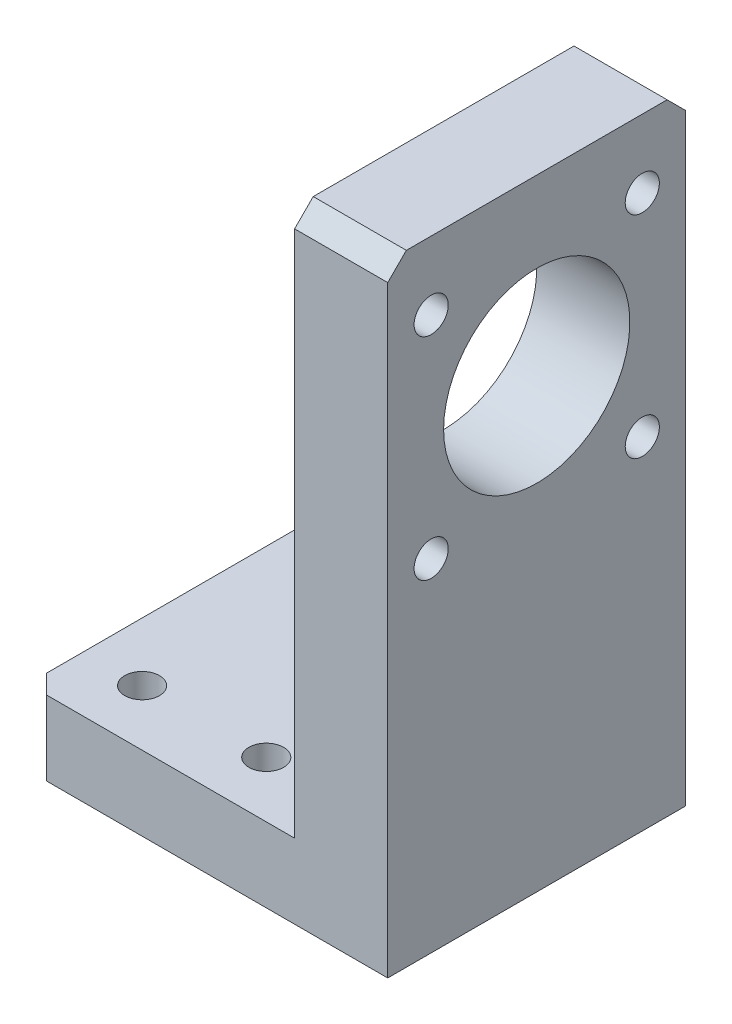
SolidWorks part; units mm, degrees
material "Q235-A"
ref_plane "Front Plane" through (0, 0, 0) normal (0, 0, 1) x (1, 0, 0)
ref_plane "Top Plane" through (0, 0, 0) normal (0, 1, 0) x (1, 0, 0)
ref_plane "Right Plane" through (0, 0, 0) normal (1, 0, 0) x (0, 0, -1)
sketch "Sketch1" plane through (0, 0, 0) normal (0, 0, 1) x (1, 0, 0)
  line L0 (-9.2474, 66.1469) -> (-9.2474, -21.8531)
  line L1 (-9.2474, -21.8531) -> (-52.2474, -21.8531)
  line L2 (-52.2474, -21.8531) -> (-52.2474, -33.8531)
  line L3 (-52.2474, -33.8531) -> (5.7526, -33.8531)
  line L4 (5.7526, -33.8531) -> (5.7526, 66.1469)
  line L5 (5.7526, 66.1469) -> (-9.2474, 66.1469)
  dimension "D1" = 58
  dimension "D2" = 100
  dimension "D3" = 12
  dimension "D4" = 15
extrude "Boss-Extrude1" add sketch "Sketch1" along normal blind 48
sketch "Sketch2" plane through (-9.2474, 0, 0) normal (-1, 0, 0) x (0, 0, 1)
  line L1 (48, -33.8531) -> (0, -33.8531) construction
  circle A0 centre (24, 38.1469) radius 15
  dimension "D1" = 72
  dimension "D2" = 30
extrude "Cut-Extrude1" cut sketch "Sketch2" against normal through all
sketch "Sketch3" plane through (-9.2474, 0, 0) normal (-1, 0, 0) x (0, 0, 1)
  line L1 (7, 21.1469) -> (41, 21.1469) construction
  line L2 (7, 21.1469) -> (7, 55.1469) construction
  line L3 (7, 55.1469) -> (41, 55.1469) construction
  line L4 (41, 21.1469) -> (41, 55.1469) construction
  line L5 (7, 21.1469) -> (41, 55.1469) construction
  line L6 (7, 55.1469) -> (41, 21.1469) construction
  point P0 (24, 38.1469)
  dimension "D1" = 34
  dimension "D2" = 34
hole_wizard "Hole size (per) hex socket cap screw type 1" positions "Sketch4" profile "Sketch5" counterbore size "M5" standard "GB" end condition through all
sketch "Sketch4" plane through (-9.2474, 0, 0) normal (-1, 0, 0) x (0, 0, 1)
  point P0 (7, 55.1469)
  point P3 (41, 55.1469)
  point P6 (41, 21.1469)
  point P9 (7, 21.1469)
sketch "Sketch5" plane through (-9.2474, 55.1469, 7) normal (0, 1, 0) x (0, 0, 1)
  line L0 (0, 0) -> (0, 15)
  line L1 (0, 15) -> (2.75, 15)
  line L3 (2.75, 15) -> (2.75, 5.7)
  line L4 (2.75, 5.7) -> (5, 5.7)
  line L5 (5, 5.7) -> (5, 0)
  line L7 (5, 0) -> (0, 0)
  line L11 (0, -6.35) -> (0, 107.95) construction
  dimension "通孔孔直径" = 5.5
  dimension "通孔孔深度" = 15
  dimension "柱形沉头孔直径" = 10
  dimension "柱形沉头孔深度" = 5.7
chamfer "Chamfer1" distance 3 angle 45 4 edges at (-52.2474, -27.8531, 48) (-52.2474, -27.8531, 0) (-1.7474, 66.1469, 48) (-1.7474, 66.1469, 0)
sketch "Sketch6" plane through (0, -21.8531, 0) normal (0, 1, 0) x (1, 0, 0)
  line L0 (-52.2474, -24) -> (5.7526, -24) construction
  line L1 (-52.2474, -45) -> (-52.2474, -3) construction
  line L2 (5.7526, -45) -> (5.7526, -3) construction
  line L4 (-42.8105, -39) -> (-22.8105, -39) construction
  line L5 (-42.8105, -39) -> (-42.8105, -9) construction
  line L6 (-42.8105, -9) -> (-22.8105, -9) construction
  line L7 (-22.8105, -39) -> (-22.8105, -9) construction
  line L8 (-42.8105, -39) -> (-22.8105, -9) construction
  line L9 (-42.8105, -9) -> (-22.8105, -39) construction
  circle A0 centre (-42.8105, -9) radius 2.8
  circle A1 centre (-22.8105, -9) radius 2.8
  circle A2 centre (-42.8105, -39) radius 2.8
  circle A3 centre (-22.8105, -39) radius 2.8
  point P6 (-32.8105, -24)
  dimension "D1" = 20
  dimension "D2" = 30
extrude "Cut-Extrude2" cut sketch "Sketch6" against normal blind 48
